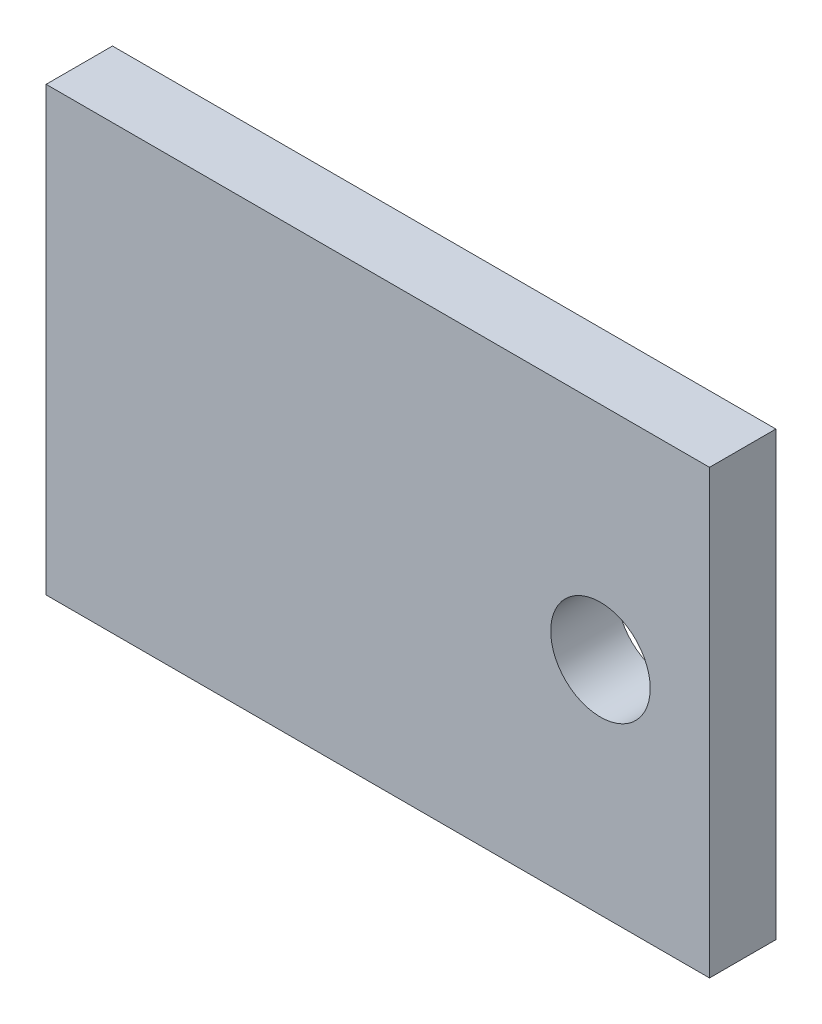
from build123d import *

# Parameters (mm, degrees)
SKETCH1_W           = 60
SKETCH1_H           = 40
BOSS_EXTRUDE1_DEPTH = 6
SKETCH2_R           = 4.5
CUT_EXTRUDE1_DEPTH  = 6


with BuildPart() as part:
    # Sketch1 → Boss-Extrude1 (new body)
    with BuildSketch(Plane.XY):
        Rectangle(SKETCH1_W, SKETCH1_H)
    extrude(amount=BOSS_EXTRUDE1_DEPTH)

    # Sketch2 → Cut-Extrude1 (cut)
    with BuildSketch(Plane.XY.offset(6)):
        with Locations((20.134545778, 0)):
            Circle(SKETCH2_R)
    extrude(amount=-CUT_EXTRUDE1_DEPTH, mode=Mode.SUBTRACT)


solid = part.part
